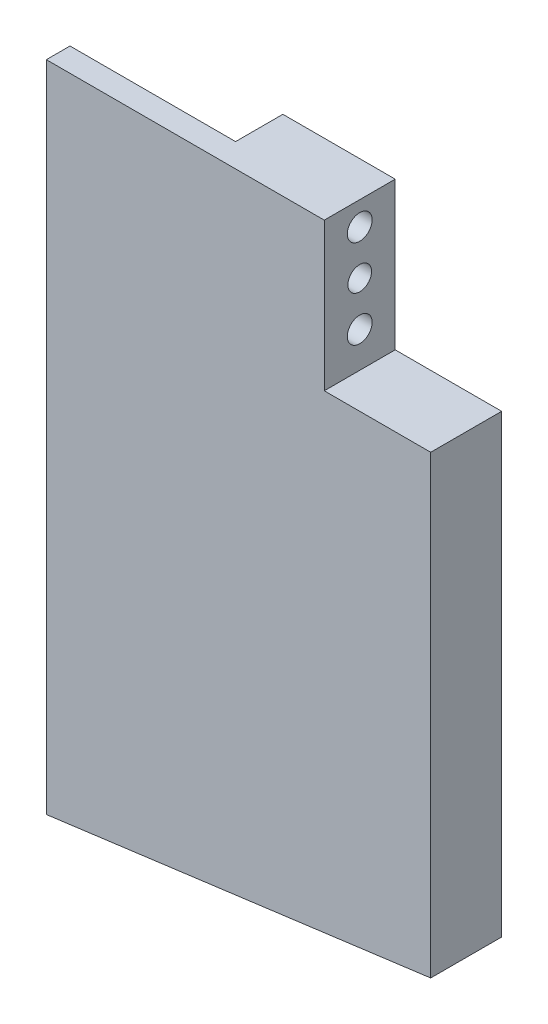
SolidWorks part; units mm, degrees
ref_plane "Front Plane" through (0, 0, 0) normal (0, 0, 1) x (1, 0, 0)
ref_plane "Top Plane" through (0, 0, 0) normal (0, 1, 0) x (1, 0, 0)
ref_plane "Right Plane" through (0, 0, 0) normal (1, 0, 0) x (0, 0, -1)
sketch "Sketch1" plane through (0, 0, 0) normal (0, 1, 0) x (1, 0, 0)
  line L1 (-32.5, 6) -> (32.5, 6)
  line L2 (-32.5, 6) -> (-32.5, -6)
  line L3 (-32.5, -6) -> (32.5, -6)
  line L4 (32.5, 6) -> (32.5, -6)
  line L5 (-32.5, 6) -> (32.5, -6) construction
  line L6 (-32.5, -6) -> (32.5, 6) construction
  point P0 (0, 0)
  dimension "D1" = 65
  dimension "D2" = 12
extrude "Boss-Extrude1" add sketch "Sketch1" along normal mid plane 102
sketch "Sketch4" plane through (0, 0, 6) normal (0, 0, 1) x (1, 0, 0)
  line L0 (-32.5, -51) -> (32.5, -51) construction
  line L1 (-32.5, -51) -> (32.5, -51)
  line L2 (32.5, -51) -> (-32.5, -59.5574)
  line L3 (-32.5, -51) -> (-32.5, -59.5574)
  dimension "D1" = 7.5
extrude "Boss-Extrude2" add sketch "Sketch4" against normal up to surface (12 mm away) up to face at (0, 0, -6)
sketch "Sketch3" plane through (0, 0, 6) normal (0, 0, 1) x (1, 0, 0)
  line L1 (32.5, 51) -> (14.5, 51)
  line L2 (32.5, 51) -> (32.5, 26)
  line L3 (32.5, 26) -> (14.5, 26)
  line L4 (14.5, 51) -> (14.5, 26)
  dimension "D1" = 25
  dimension "D2" = 18
extrude "Cut-Extrude2" cut sketch "Sketch3" against normal through all
hole_wizard "M5 Tapped Hole1" positions "Sketch6" profile "Sketch5" tap size "M5" standard "Gb"
sketch "Sketch6" plane through (7.1536, -54.3369, 0) normal (0.1305, -0.9914, 0) x (-0.9914, -0.1305, 0)
  line L0 (-25.5651, -6) -> (-25.5651, 6) construction
  point P0 (-18.0651, 0)
  point P2 (6.9349, 0)
  point P4 (31.9349, 0)
  dimension "D1" = 25
  dimension "D2" = 25
  dimension "D3" = 7.5
sketch "Sketch5" plane through (25.0642, -51.9789, 0) normal (0, 0, 1) x (0.9914, 0.1305, 0)
  line L0 (0, 0) -> (0, 13.6618)
  line L1 (0, 13.6618) -> (2.1, 12.4)
  line L2 (2.1, 12.4) -> (2.1, 0)
  line L5 (2.1, 0) -> (0, 0)
  line L10 (0, 13.6618) -> (-2.1, 12.4) construction
  line L11 (0, -6.35) -> (0, 107.95) construction
  dimension "螺纹孔钻头直径" = 4.2
  dimension "螺纹孔钻头深度" = 12.4
  dimension "导头角度" = 118
cosmetic thread "Hole Thread2" parameters "D1"=10, "D2"=5
cosmetic thread "Hole Thread3" parameters "D1"=10, "D2"=5
cosmetic thread "Hole Thread4" parameters "D1"=10, "D2"=5
hole_wizard "M5 Tapped Hole2" positions "Sketch8" profile "Sketch7" tap size "M5" standard "Gb"
sketch "Sketch8" plane through (-32.5, 0, 0) normal (-1, 0, 0) x (0, 0, 1)
  line L0 (-6, 51) -> (6, 51) construction
  point P0 (0, 43)
  point P2 (0, 3)
  point P4 (0, -37)
  dimension "D1" = 8
  dimension "D2" = 40
  dimension "D3" = 40
sketch "Sketch7" plane through (-32.5, 43, 0) normal (0, 1, 0) x (0, 0, 1)
  line L0 (0, 0) -> (0, 13.6618)
  line L1 (0, 13.6618) -> (2.1, 12.4)
  line L2 (2.1, 12.4) -> (2.1, 0)
  line L5 (2.1, 0) -> (0, 0)
  line L10 (0, 13.6618) -> (-2.1, 12.4) construction
  line L11 (0, -6.35) -> (0, 107.95) construction
  dimension "螺纹孔钻头直径" = 4.2
  dimension "螺纹孔钻头深度" = 12.4
  dimension "导头角度" = 118
cosmetic thread "Hole Thread5" parameters "D1"=10, "D2"=5
cosmetic thread "Hole Thread6" parameters "D1"=10, "D2"=5
cosmetic thread "Hole Thread7" parameters "D1"=10, "D2"=5
hole_wizard "M5 Tapped Hole3" positions "Sketch10" profile "Sketch9" tap size "M5" standard "Gb"
sketch "Sketch10" plane through (14.5, 0, 0) normal (1, 0, 0) x (0, 0, -1)
  line L0 (6, 51) -> (-6, 51) construction
  point P0 (0, 47)
  point P2 (0, 32)
  dimension "D1" = 4
  dimension "D2" = 15
sketch "Sketch9" plane through (14.5, 47, 0) normal (0, 1, 0) x (0, 0, -1)
  line L0 (0, 0) -> (0, 13.6618)
  line L1 (0, 13.6618) -> (2.1, 12.4)
  line L2 (2.1, 12.4) -> (2.1, 0)
  line L5 (2.1, 0) -> (0, 0)
  line L10 (0, 13.6618) -> (-2.1, 12.4) construction
  line L11 (0, -6.35) -> (0, 107.95) construction
  dimension "螺纹孔钻头直径" = 4.2
  dimension "螺纹孔钻头深度" = 12.4
  dimension "导头角度" = 118
cosmetic thread "Hole Thread8" parameters "D1"=10, "D2"=5
cosmetic thread "Hole Thread9" parameters "D1"=10, "D2"=5
sketch "Sketch12" plane through (-32.5, 0, 0) normal (-1, 0, 0) x (0, 0, 1)
  line L0 (-6, 43) -> (-6, 51)
  line L1 (-6, 51) -> (2, 51)
  line L2 (2, 51) -> (-6, 43)
  line L3 (-6, 51) -> (6, 51) construction
  line L4 (-6, 51) -> (-6, -59.5574) construction
  dimension "D1" = 45
  dimension "D2" = 8
extrude "Cut-Extrude3" cut sketch "Sketch12" against normal blind 28
hole_wizard "Ø4.0 (4) Diameter Hole1" positions "Sketch14" profile "Sketch13" hole size "Ø4.0" standard "Gb"
sketch "Sketch14" plane through (14.5, 0, 0) normal (1, 0, 0) x (0, 0, -1)
  circle A0 centre (0, 32) radius 2.1 construction
  point P0 (0, 39.5)
  dimension "D1" = 7.5
sketch "Sketch13" plane through (14.5, 39.5, 0) normal (0, 1, 0) x (0, 0, -1)
  line L0 (0, 0) -> (0, 9.2017)
  line L1 (0, 9.2017) -> (2, 8)
  line L2 (2, 8) -> (2, 0)
  line L5 (2, 0) -> (0, 0)
  line L10 (0, 9.2017) -> (-2, 8) construction
  line L11 (0, -6.35) -> (0, 107.95) construction
  dimension "孔直径" = 4
  dimension "孔深度" = 8
  dimension "导头角度" = 118
